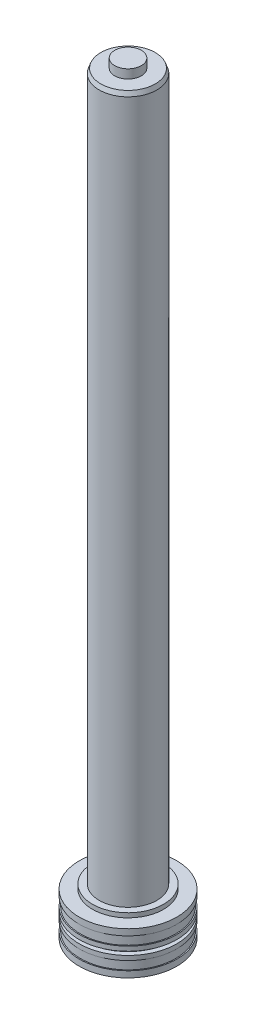
from build123d import *


with BuildPart() as part:
    # Sketch1 → Revolve1 (revolve)
    with BuildSketch(Plane.XY, mode=Mode.PRIVATE) as revolve1_sk:
        Polygon((0, 0), (80, 0), (80, 9.9), (110, 9.9), (110, 23.9), (107.5, 23.9), (107.5, 43.9), (110, 43.9), (110, 53.9), (99.5, 53.9), (99.5, 62), (110, 62), (110, 72), (107.5, 72), (107.5, 92), (110, 92), (110, 106), (80, 106), (80, 116), (65, 116), (65, 1698), (61.360297657, 1708), (30, 1708), (30, 1728), (0, 1728), align=None)
    revolve(revolve1_sk.sketch.rotate(Axis((0, 0, 0), (0, 1, 0)), 90), axis=Axis((0, 0, 0), (0, 1, 0)))


solid = part.part
